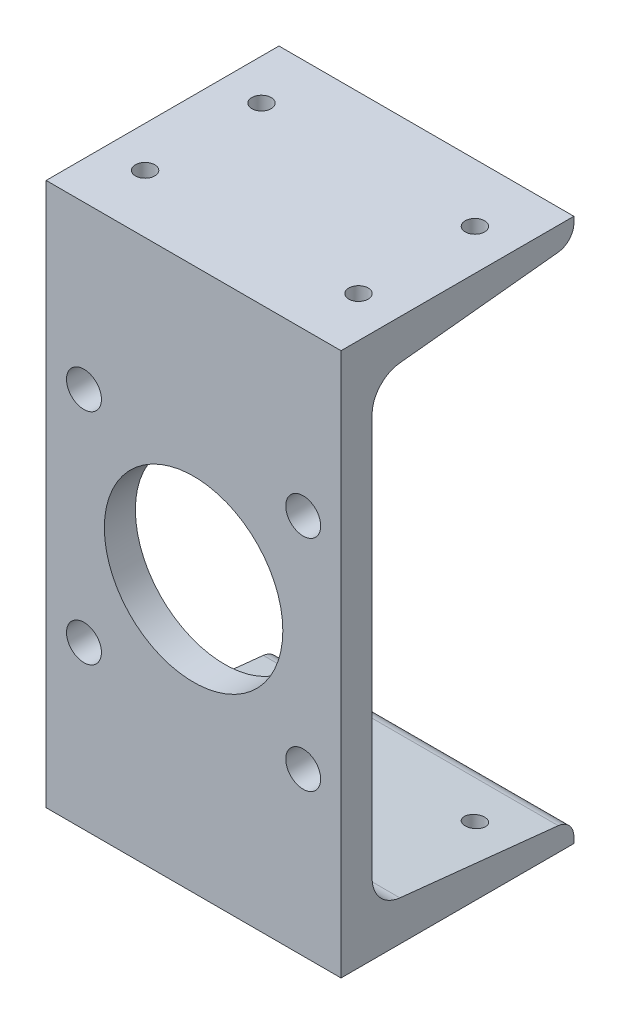
from build123d import *

# Parameters (mm, degrees)
MEMBER_1_DEPTH      = 76
SKETCH_4_R          = 23
CUT_EXTRUDE_1_DEPTH = 171.223382648
SKETCH_6_R          = 4.5
CUT_EXTRUDE_2_DEPTH = 171.223382648
HOLE_WIZARD_M6_1_D  = 5


with BuildPart() as part:
    # Sketch11 → Member 1 (new body)
    with BuildSketch(Plane(origin=(0, 0, 0), x_dir=(0, 0, -1), z_dir=(1, 0, 0))):
        with BuildLine():
            Line((60, 140), (0, 140))
            Line((0, 140), (0, 0))
            Line((0, 0), (60, 0))
            Line((60, 0), (60, 1.539529212))
            ThreePointArc((60, 1.539529212), (58.844151715, 4.550616941), (55.970378085, 6.014877742))
            Line((55.970378085, 6.014877742), (15.163772294, 10.303824837))
            ThreePointArc((15.163772294, 10.303824837), (10.054841396, 12.906955149), (8, 18.26))
            Line((8, 18.26), (8, 121.74))
            ThreePointArc((8, 121.74), (10.054841396, 127.093044851), (15.163772294, 129.696175163))
            Line((15.163772294, 129.696175163), (55.970378085, 133.985122258))
            ThreePointArc((55.970378085, 133.985122258), (58.844151715, 135.449383059), (60, 138.460470788))
            Line((60, 138.460470788), (60, 140))
        make_face()
    extrude(amount=MEMBER_1_DEPTH)

    # 草图4 → 切除-拉伸1 (cut, through all)
    with BuildSketch(Plane.XY):
        with Locations((38, 70)):
            Circle(SKETCH_4_R)
    extrude(amount=-CUT_EXTRUDE_1_DEPTH, mode=Mode.SUBTRACT)

    # 草图6 → 切除-拉伸2 (cut, through all)
    with BuildSketch(Plane.XY):
        with Locations((66.25, 41.75)):
            Circle(SKETCH_6_R)
        with Locations((9.75, 41.75)):
            Circle(SKETCH_6_R)
        with Locations((66.25, 98.25)):
            Circle(SKETCH_6_R)
        with Locations((9.75, 98.25)):
            Circle(SKETCH_6_R)
    extrude(amount=-CUT_EXTRUDE_2_DEPTH, mode=Mode.SUBTRACT)

    # M6 螺纹孔1 (through all)
    with Locations(Plane(origin=(0, 0, 0), x_dir=(-1, 0, 0), z_dir=(0, -1, 0))):
        with Locations((-65.5, 15), (-65.5, 45), (-10.5, 15), (-10.5, 45)):
            Hole(HOLE_WIZARD_M6_1_D / 2)


solid = part.part
